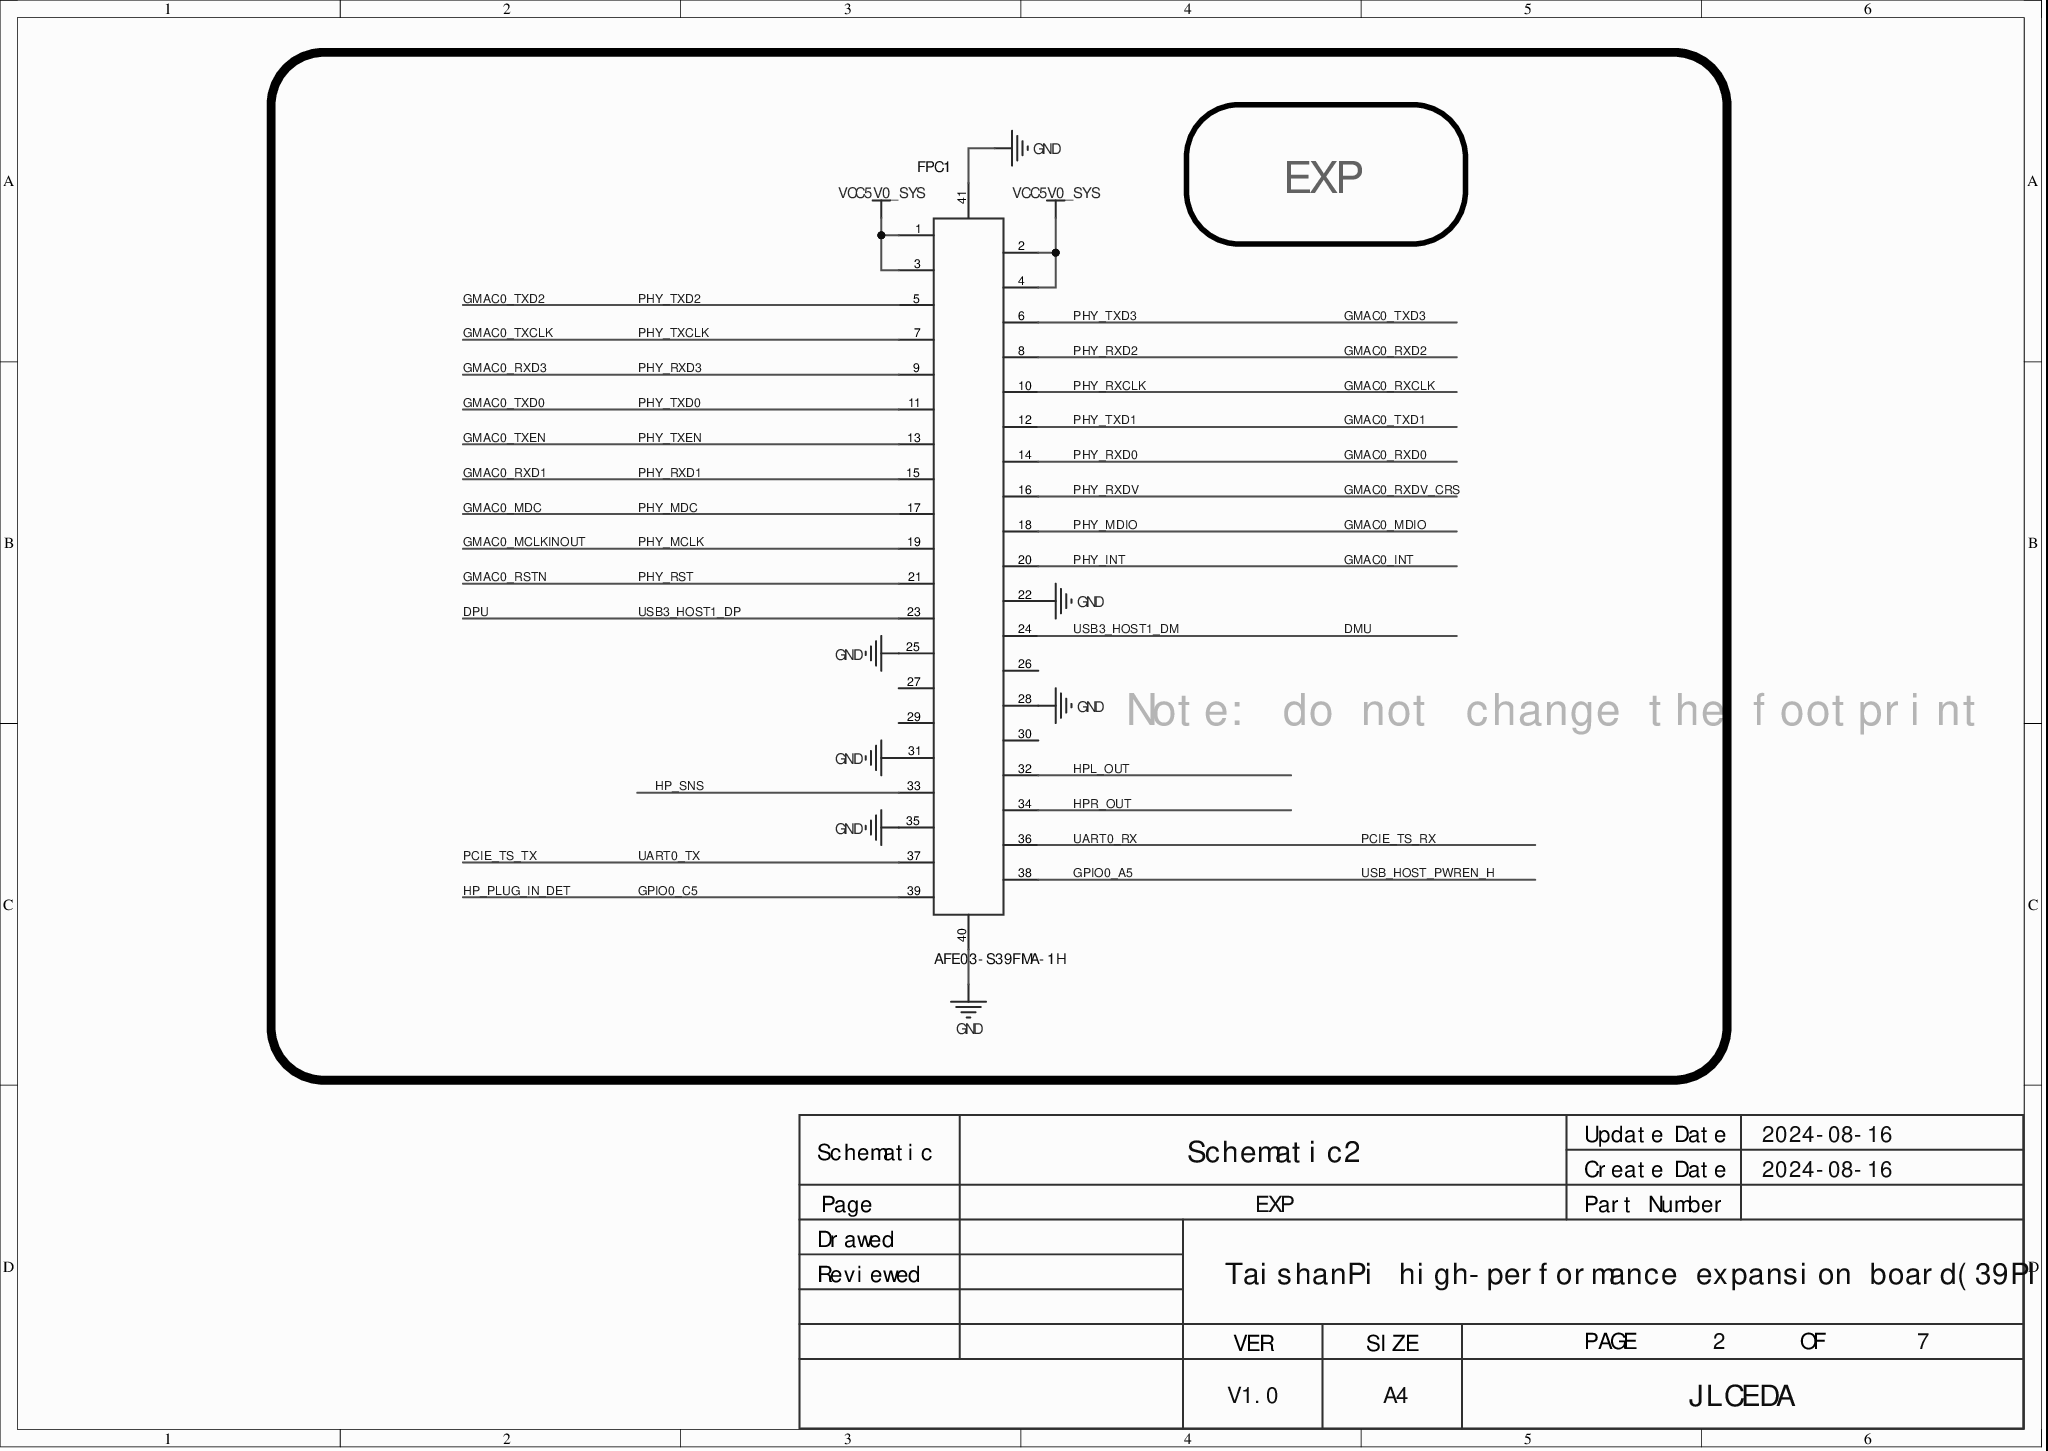
[diagram p0: MISC84334-2.SchDoc]
# Altium project MISC84334.PrjPcb (part 1 of 5)
7 sheets, 209 parts. Net scope: global (net labels, ports and power ports of the same name join across sheets).
Board file: MISC84334.PcbDoc
Sheets:
  MISC84334-2.SchDoc
  MISC84334-3.SchDoc
  MISC84334-4.SchDoc
  MISC84334-5.SchDoc
  MISC84334-6.SchDoc
  MISC84334-7.SchDoc
  MISC84334-8.SchDoc

## Sheet MISC84334-2.SchDoc
size 297 x 210 mm; Symbol: Sheet-Symbol_A4; Company: JLCEDA; Version: V1.0; Page Size: A4; @Project Name: COMPANY_A TaishanPi high-performance expansion board(39PIN); @Page Count: 7; @Update Date: 2024-08-16; @Create Date: 2024-08-16; @Schematic Name: Schematic2; @Page No: 2; @Page Name: EXP; Device: Sheet-Symbol_A4

### Parts
FPC1  AFE03-S39FMA-1H  [FPC-SMD_P0.30-39P_FGS-XJ-H1.0]

### Nets
GND: FPC1.22 FPC1.25 FPC1.28 FPC1.31 FPC1.35 FPC1.40 FPC1.41
VCC5V0_SYS: FPC1.1 FPC1.2 FPC1.3 FPC1.4
DMU: FPC1.24  [also labelled USB3_HOST1_DM]
DPU: FPC1.23  [also labelled USB3_HOST1_DP]
GMAC0_INT: FPC1.20  [also labelled PHY_INT]
GMAC0_MCLKINOUT: FPC1.19  [also labelled PHY_MCLK]
GMAC0_MDC: FPC1.17  [also labelled PHY_MDC]
GMAC0_MDIO: FPC1.18  [also labelled PHY_MDIO]
GMAC0_RSTN: FPC1.21  [also labelled PHY_RST]
GMAC0_RXCLK: FPC1.10  [also labelled PHY_RXCLK]
GMAC0_RXD0: FPC1.14  [also labelled PHY_RXD0]
GMAC0_RXD1: FPC1.15  [also labelled PHY_RXD1]
GMAC0_RXD2: FPC1.8  [also labelled PHY_RXD2]
GMAC0_RXD3: FPC1.9  [also labelled PHY_RXD3]
GMAC0_RXDV_CRS: FPC1.16  [also labelled PHY_RXDV]
GMAC0_TXCLK: FPC1.7  [also labelled PHY_TXCLK]
GMAC0_TXD0: FPC1.11  [also labelled PHY_TXD0]
GMAC0_TXD1: FPC1.12  [also labelled PHY_TXD1]
GMAC0_TXD2: FPC1.5  [also labelled PHY_TXD2]
GMAC0_TXD3: FPC1.6  [also labelled PHY_TXD3]
GMAC0_TXEN: FPC1.13  [also labelled PHY_TXEN]
GPIO0_A5: FPC1.38  [also labelled USB_HOST_PWREN_H]
GPIO0_C5: FPC1.39  [also labelled HP_PLUG_IN_DET]
HP_SNS: FPC1.33
HPL_OUT: FPC1.32
HPR_OUT: FPC1.34
PCIE_TS_RX: FPC1.36  [also labelled UART0_RX]
PCIE_TS_TX: FPC1.37  [also labelled UART0_TX]

Not connected (* = marked no-connect by the designer): FPC1 26 27 29 30

### Notes on the sheet
- EXP
- Note: do not change the footprint
- Update Date
- 2024-08-16
- Schematic
- Page
- Schematic2
- Create Date
- Part Number
- Reviewed
- Drawed
- COMPANY_A TaishanPi high-performance expansion board(39PIN)
- VER
- V1.0
- SIZE
- A4
- PAGE
- 2
- JLCEDA
- OF
- 7

### Library data of the parts
FPC1 = AFE03-S39FMA-1H: Pitch:0.3mm;Contacts:39;Locking:Flip lock;Mounting type:Horizontal SMD;Contact type:Bottom contact;; Manufacturer: JS(钜硕电子); AddInBom: yes; Pitch: 0.3mm; Number of Contacts: 39; FFC, FCB Thickness: 0.2mm; ModelId: 90cc611c06ba4f59bb65cf3349ad002a; ModelTransform: 523.621,133.858,0,180,0,0,0.018,-4.843,0; Symbol: AFE03-S39FMA-1H; Device: AFE03-S39FMA-1H; LCSC Part Name: 0.3mm P数:39 翻盖式 下接; SupplierPart: C262546; ManufacturerPart: AFE03-S39FMA-1H; Supplier Footprint: SMD,P=0.3mm; Datasheet: https://atta.szlcsc.com/upload/public/pdf/source/20180810/C262546_FD07BEB9163FBD4C911947212CF39B0D.pdf; Supplier: LCSC; ConvertToPcb: yes; Locking Feature: Flip lock; Mounting Type: Horizontal SMD; Contact Type: Bottom contact; Height Above Board: 1mm; FootprintName: FPC-SMD_P0.30-39P_FGS-XJ-H1.0; ModelName: FPC-SMD_P0.30-39P_FGS-XJ-H1.0

## Sheet MISC84334-3.SchDoc
size 297 x 210 mm; Symbol: Sheet-Symbol_A4; Company: JLCEDA; Version: V1.0; Page Size: A4; @Project Name: COMPANY_A TaishanPi high-performance expansion board(39PIN); @Page Count: 7; @Update Date: 2024-08-16; @Create Date: 2024-08-16; @Schematic Name: Schematic2; @Page No: 4; @Page Name: FE2.1; Device: Sheet-Symbol_A4
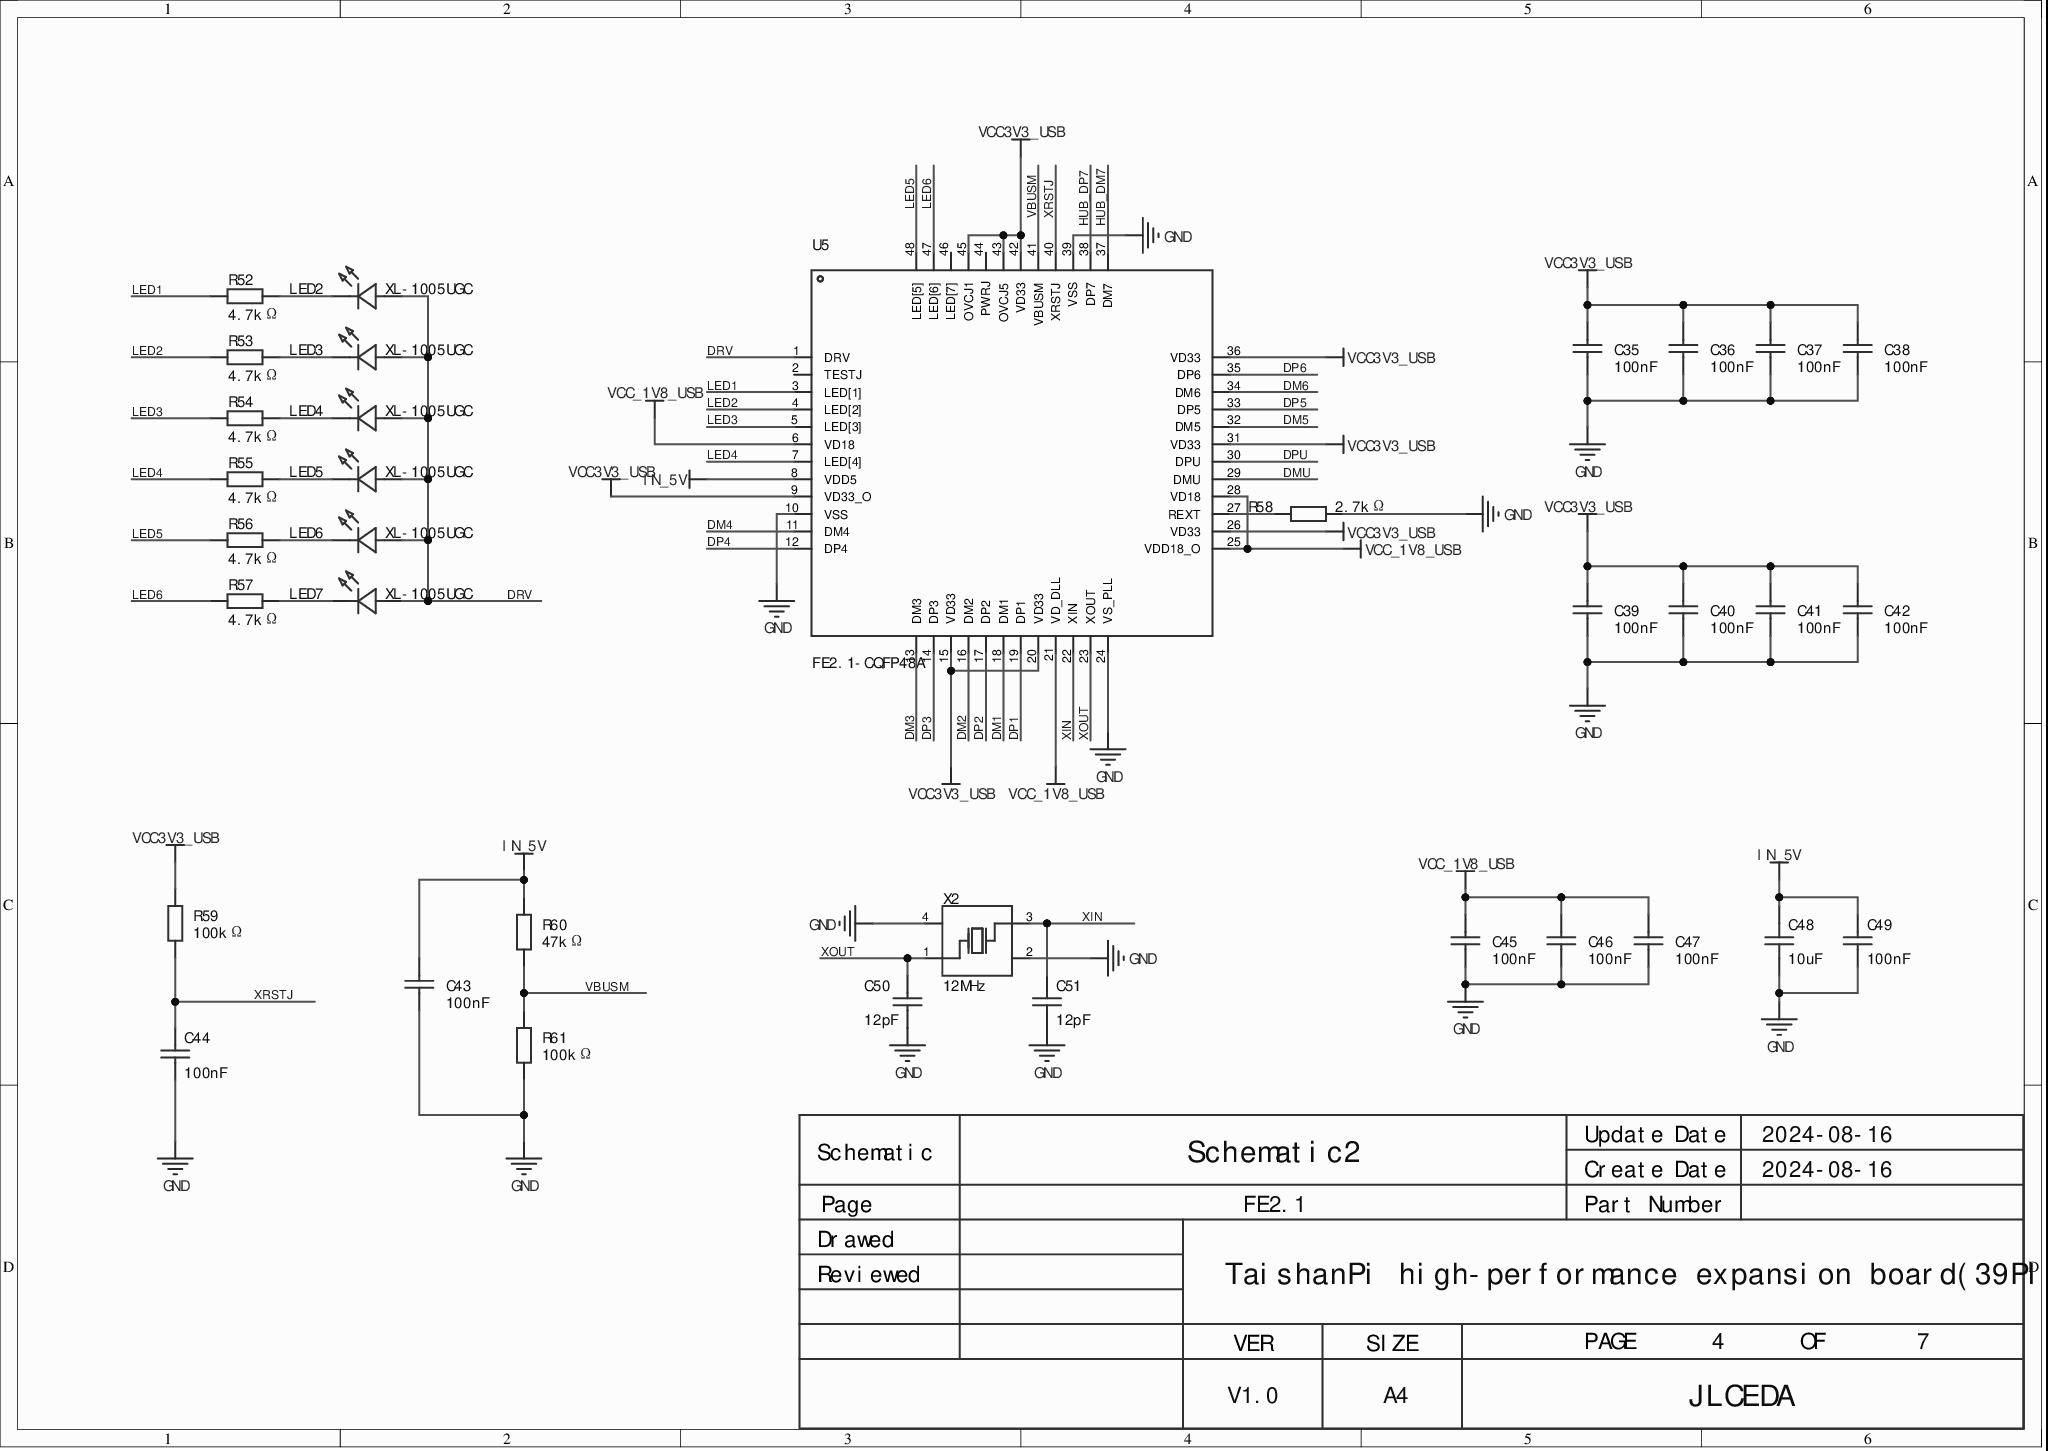
[diagram p1: MISC84334-3.SchDoc]

### Parts
C35  100nF  [R0402]
C36  100nF  [R0402]
C37  100nF  [R0402]
C38  100nF  [R0402]
C39  100nF  [R0402]
C40  100nF  [R0402]
C41  100nF  [R0402]
C42  100nF  [R0402]
C43  100nF  [R0402]
C44  100nF  [R0402]
C45  100nF  [R0402]
C46  100nF  [R0402]
C47  100nF  [R0402]
C48  10uF  [r0603]
C49  100nF  [R0402]
C50  12pF  [R0402]
C51  12pF  [R0402]
LED2  XL-1005UGC  [LED0402-RD_GREEN]
LED3  XL-1005UGC  [LED0402-RD_GREEN]
LED4  XL-1005UGC  [LED0402-RD_GREEN]
LED5  XL-1005UGC  [LED0402-RD_GREEN]
LED6  XL-1005UGC  [LED0402-RD_GREEN]
LED7  XL-1005UGC  [LED0402-RD_GREEN]
R52  4.7kΩ  [R0402]
R53  4.7kΩ  [R0402]
R54  4.7kΩ  [R0402]
R55  4.7kΩ  [R0402]
R56  4.7kΩ  [R0402]
R57  4.7kΩ  [R0402]
R58  2.7kΩ  [R0402]
R59  100kΩ  [R0402]
R60  47kΩ  [R0402]
R61  100kΩ  [R0402]
U5  FE2.1-CQFP48A  [LQFP-48_L7.0-W7.0-P0.50-LS9.0-BL]
X2  12MHz  [OSC-SMD_4P-L3.2-W2.5-BL]

### Nets
GND: C35.1 C36.1 C37.1 C38.1 C39.1 C40.1 C41.1 C42.1 C43.1 C44.1 C45.1 C46.1 C47.1 C48.1 C49.1 C50.1 C51.2 R58.2 R61.1 U5.10(VSS) U5.24(VS_PLL) U5.39(VSS) X2.2(GND) X2.4(GND)
IN_5V: C43.2 C48.2 C49.2 R60.2 U5.8(VDD5)
VCC3V3_USB: C35.2 C36.2 C37.2 C38.2 C39.2 C40.2 C41.2 C42.2 R59.2 U5.9(VD33_O) U5.15(VD33) U5.20(VD33) U5.26(VD33) U5.31(VD33) U5.36(VD33) U5.42(VD33) U5.43(OVCJ5) U5.45(OVCJ1)
VCC_1V8_USB: C45.2 C46.2 C47.2 U5.6(VD18) U5.21(VD_DLL) U5.25(VDD18_O) U5.28(VD18)
DM1: U5.18(DM1)
DM2: U5.16(DM2)
DM3: U5.13(DM3)
DM4: U5.11(DM4)
DM5: U5.32(DM5)
DM6: U5.34(DM6)
DMU: U5.29(DMU)
DP1: U5.19(DP1)
DP2: U5.17(DP2)
DP3: U5.14(DP3)
DP4: U5.12(DP4)
DP5: U5.33(DP5)
DP6: U5.35(DP6)
DPU: U5.30(DPU)
DRV: LED2.2(A) LED3.2(A) LED4.2(A) LED5.2(A) LED6.2(A) LED7.2(A) U5.1(DRV)
HUB_DM7: U5.37(DM7)
HUB_DP7: U5.38(DP7)
LED1: R52.2 U5.3(LED[1])
LED2: R53.2 U5.4(LED[2])
LED3: R54.2 U5.5(LED[3])
LED4: R55.2 U5.7(LED[4])
LED5: R56.2 U5.48(LED[5])
LED6: R57.2 U5.47(LED[6])
VBUSM: R60.1 R61.2 U5.41(VBUSM)
XIN: C51.1 U5.22(XIN) X2.3(OSC2)
XOUT: C50.2 U5.23(XOUT) X2.1(OSC1)
XRSTJ: C44.2 R59.1 U5.40(XRSTJ)
NetLED2_1: LED2.1(K) R52.1
NetLED3_1: LED3.1(K) R53.1
NetLED4_1: LED4.1(K) R54.1
NetLED5_1: LED5.1(K) R55.1
NetLED6_1: LED6.1(K) R56.1
NetLED7_1: LED7.1(K) R57.1
NetR58_1: R58.1 U5.27(REXT)

Not connected (* = marked no-connect by the designer): U5 2(TESTJ)* 44(PWRJ)* 46(LED[7])*

### Notes on the sheet
- Update Date
- 2024-08-16
- Schematic
- Page
- Schematic2
- FE2.1
- Create Date
- Part Number
- Reviewed
- Drawed
- COMPANY_A TaishanPi high-performance expansion board(39PIN)
- VER
- V1.0
- SIZE
- A4
- PAGE
- 4
- JLCEDA
- OF
- 7

### Library data of the parts
C35-C47 C49 = CL05B104KO5NNNC: Capacitance:100nF;Tolerance:±10%;Rated voltage:16V;Dielectric(Temp. coefficient):X7R;; Manufacturer: SAMSUNG(三星); AddInBom: yes; ModelId: 36a51122f27c49738f86b3bfa98863e0; ModelName: C0402_L1.0-W0.5-H0.5; ModelTransform: 39.37,19.685,0,0,0,0,0,0,0; Tolerance: ±10%; Voltage Rated: 16V; Temperature Coefficient: X7R; Symbol: CL05B104KO5NNNC; Device: CL05B104KO5NNNC; LCSC Part Name: 100nF ±10% 16V; SupplierPart: C1525; ManufacturerPart: CL05B104KO5NNNC; Supplier Footprint: 0402; JLCPCB Part Class: Basic library; Datasheet: https://atta.szlcsc.com/upload/public/pdf/source/20160103/1457707674891.pdf; Supplier: LCSC; ConvertToPcb: yes; FootprintName: R0402; Value: 100nF
C48 = 0603X106M100CT: Capacitance:10uF;Tolerance:±20%;Rated voltage:10V;Dielectric(Temp. coefficient):X5R;; Manufacturer: Walsin(华新科); AddInBom: yes; ModelId: ac125912035d415993ca9572d50418b1; ModelName: C0603_L1.6-W0.8-H0.8; ModelTransform: 62.992,31.496,0,0,0,0,0,0,0; Tolerance: ±20%; Voltage Rated: 10V; Temperature Coefficient: X5R; Symbol: 0603X106M100; Device: 0603X106M100CT; LCSC Part Name: 10uF ±20% 10V; SupplierPart: C89283; ManufacturerPart: 0603X106M100CT; Supplier Footprint: 0603; JLCPCB Part Class: Extended library; Datasheet: https://atta.szlcsc.com/upload/public/pdf/source/20161226/1482720147964.pdf; Supplier: LCSC; ConvertToPcb: yes; FootprintName: r0603; Value: 10uF
C50 C51 = 0402CG120J500NT: Capacitance:12pF;Tolerance:±5%;Rated voltage:50V;Dielectric(Temp. coefficient):C0G;; Manufacturer: FH(风华); Symbol: 0402CG200J500NT; Capacitance: 20pF; AddInBom: yes; ModelId: 36a51122f27c49738f86b3bfa98863e0; ModelName: C0402_L1.0-W0.5-H0.5; ModelTransform: 39.37,19.685,0,0,0,0,0,0,0; Tolerance: ±5%; Voltage Rated: 50V; Temperature Coefficient: C0G; JLCPCB Part Class: Basic Part; Device: 0402CG120J500NT; Supplier: LCSC; Manufacturer Part: 0402CG120J500NT; Supplier Part: C1547; LCSC Part Name: 12pF ±5% 50V; Supplier Footprint: 0402; Datasheet: https://atta.szlcsc.com/upload/public/pdf/source/20200305/C486355_26A10D38EF8C2A5C37091D0039909270.pdf; ConvertToPcb: yes; FootprintName: R0402; Value: 12pF
LED2-LED7 = XL-1005UGC: Emitting color:Emerald green;Dominant wavelength:516nm;Color temp.:-;Power:80mW;Mounting:Top mount;; Manufacturer: XINGLIGHT(成兴光); Symbol: XL-1005UGC_C2856703; AddInBom: yes; ModelId: 080bb9bd520f4b34ac21e218e7b036d6; ModelName: LED0402_L1.0-W0.5-H0.2; ModelTransform: 40.1574,19.685,0,0,0,0,0,-0.0005,0; Lens Color: Water clear; Dominant Wavelength: 516nm; Peak Wavelength: 531nm; Forward Current: 25mA; Power Dissipation: 80mW; Viewing Angle: 120°; Device: XL-1005UGC; LCSC Part Name: 正贴; SupplierPart: C2856703; ManufacturerPart: XL-1005UGC; Supplier Footprint: 0402; Datasheet: https://atta.szlcsc.com/upload/public/pdf/source/20221102/FF8D6BC2225363A60A01D46BB802F217.pdf; Supplier: LCSC; ConvertToPcb: yes; FootprintName: LED0402-RD_GREEN; Emitted Color: Emerald green; Color Temperature: -; Mounting Sytle: Top mount; Operating Temperature: -30℃~+85℃
R52-R57 = 0402WGF4701TCE: Resistor type:Thick film resistor;Resistance:4.7kΩ;Tolerance:±1%;Power:62.5mW;; Manufacturer: UNI-ROYAL(厚声); AddInBom: yes; ModelId: 671aefced39d4c318694bba8bd8efd39; ModelName: R0402_L1.0-W0.5-H0.5; ModelTransform: 39.37,19.685,0,0,0,0,0,0.0005,0; Tolerance: ±1%; Power(Watts): 62.5mW; Temperature Coefficient: ±100ppm/℃; Overload Voltage (Max): 50V; Symbol: 0402WGF4701TCE; Device: 0402WGF4701TCE; Supplier: LCSC; Manufacturer Part: 0402WGF4701TCE; Supplier Part: C25900; Value: 4.7kΩ; JLCPCB Part Class: Basic library; LCSC Part Name: 4.7kΩ ±1% 62.5mW; Supplier Footprint: 0402; Datasheet: https://atta.szlcsc.com/upload/public/pdf/source/20200306/C422600_1E6D84923E4A46A82E41ADD87F860B5C.pdf; ConvertToPcb: yes; FootprintName: R0402; Type: Thick film resistor; Operating Temperature Range: -55℃~+155℃
R58 = RC0402FR-072K7L: Resistor type:Thick film resistor;Resistance:2.7kΩ;Tolerance:±1%;Power:62.5mW;; Manufacturer: YAGEO(国巨); AddInBom: yes; ModelId: 671aefced39d4c318694bba8bd8efd39; ModelName: R0402_L1.0-W0.5-H0.5; ModelTransform: 39.37,19.685,0,0,0,0,0,0.0005,0; Tolerance: ±1%; Power(Watts): 62.5mW; Temperature Coefficient: ±100ppm/℃; Overload Voltage (Max): 50V; Symbol: RC0402FR-072K7L; Device: RC0402FR-072K7L; LCSC Part Name: 2.7kΩ ±1% 62.5mW; SupplierPart: C138017; ManufacturerPart: RC0402FR-072K7L; Supplier Footprint: 0402; Datasheet: https://atta.szlcsc.com/upload/public/pdf/source/20171107/C138017_15100516423651096944.pdf; Supplier: LCSC; ConvertToPcb: yes; FootprintName: R0402; Type: Thick film resistor; Value: 2.7kΩ; Operating Temperature Range: -55℃~+155℃
R59 R61 = 0402WGF1003TCE: Resistor type:Thick film resistor;Resistance:100kΩ;Tolerance:±1%;Power:62.5mW;Temp. coefficient:±100ppm/℃;Max working voltage:50V;Operating temperature:-55℃~+155℃;; Manufacturer: UNI-ROYAL(厚声); AddInBom: yes; ModelId: 671aefced39d4c318694bba8bd8efd39; ModelName: R0402_L1.0-W0.5-H0.5; ModelTransform: 39.37,19.685,0,0,0,0,0,0.0005,0; Tolerance: ±1%; Power(Watts): 62.5mW; Overload Voltage (Max): 50V; Symbol: 0402WGF1003TCE; Device: 0402WGF1003TCE; LCSC Part Name: 100kΩ ±1% 62.5mW; SupplierPart: C25741; ManufacturerPart: 0402WGF1003TCE; Supplier Footprint: 0402; JLCPCB Part Class: Basic Part; Datasheet: https://atta.szlcsc.com/upload/public/pdf/source/20200306/C422600_1E6D84923E4A46A82E41ADD87F860B5C.pdf; Supplier: LCSC; ConvertToPcb: yes; FootprintName: R0402; Type: Thick film resistor; Value: 100kΩ; Temperature Coefficient: ±100ppm/℃; Operating Temperature Range: -55℃~+155℃
R60 = 0402WGF4702TCE: Resistor type:Thick film resistor;Resistance:47kΩ;Tolerance:±1%;Power:62.5mW;; Manufacturer: UNI-ROYAL(厚声); AddInBom: yes; ModelId: 671aefced39d4c318694bba8bd8efd39; ModelName: R0402_L1.0-W0.5-H0.5; ModelTransform: 39.37,19.685,0,0,0,0,0,0.0005,0; Tolerance: ±1%; Power(Watts): 62.5mW; Temperature Coefficient: ±100ppm/℃; Overload Voltage (Max): 50V; Symbol: 0402WGF4702TCE; Device: 0402WGF4702TCE; LCSC Part Name: 47kΩ ±1% 62.5mW; SupplierPart: C25792; ManufacturerPart: 0402WGF4702TCE; Supplier Footprint: 0402; Datasheet: https://atta.szlcsc.com/upload/public/pdf/source/20200306/C422600_1E6D84923E4A46A82E41ADD87F860B5C.pdf; Supplier: LCSC; ConvertToPcb: yes; FootprintName: R0402; Type: Thick film resistor; Value: 47kΩ; Operating Temperature Range: -55℃~+155℃
U5 = FE2.1-CQFP48A: Type:-;Protocol:-;Drivers/receivers:-;Data rate:-;; Manufacturer: TERMINUS; Symbol: FE2.1; AddInBom: yes; ModelId: 093be70396ff421eb2cdb946d5311efc; ModelName: LQFP-48_L7.0-W7.0-H1.4-LS9.0-P0.50; ModelTransform: 354.331,354.331,0,0,0,0,0,0,0; Device: FE2.1-CQFP48A; LCSC Part Name: FE2.1-CQFP48A; SupplierPart: C39693; ManufacturerPart: FE2.1-CQFP48A; Supplier Footprint: LQFP-48(7x7); Datasheet: https://atta.szlcsc.com/upload/public/pdf/source/20220804/15245222ED887981AE0D8A621FDC31A4.pdf; Supplier: LCSC; ConvertToPcb: yes; FootprintName: LQFP-48_L7.0-W7.0-P0.50-LS9.0-BL; Type: -; Protocol: -; Number of Drivers/Receivers: -; Data Rate: -; Supply Voltage: -
X2 = X322512MSB4SI: Frequency:12MHz;Frequency tolerance:±10ppm;Load capacitance:20pF;; Manufacturer: YXC(扬兴晶振); AddInBom: yes; ModelId: ae22b8d143894765bc8100c37cb6356f; ModelName: OSC-SMD_4P-L3.2-W2.5-H1.0; ModelTransform: 125.984,98.425,0,0,0,0,0,0,0; Crystal Type: SMD passive crystal; Frequency Tolerance: ±10ppm; Frequency Stability: ±30ppm; Load Capacitance: 20pF; Symbol: X322512MSB4SI; Device: X322512MSB4SI; LCSC Part Name: 12MHz ±10ppm 20pF YSX321SL; SupplierPart: C9002; ManufacturerPart: X322512MSB4SI; Supplier Footprint: SMD3225-4P; Datasheet: https://atta.szlcsc.com/upload/public/pdf/source/20210329/C112971_1F611BDC486E193C1706F6D8EB5AA189.pdf; Supplier: LCSC; ConvertToPcb: yes; FootprintName: OSC-SMD_4P-L3.2-W2.5-BL; Value: 12MHz; Operating Temperature: -40℃~+85℃

## Sheet MISC84334-4.SchDoc
size 297 x 210 mm; Symbol: Sheet-Symbol_A4; Company: JLCEDA; Version: V1.0; Page Size: A4; @Project Name: COMPANY_A TaishanPi bottom 39Pin_Hub2.0_Ethernet expansion board 0419 revision; @Page Count: 7; @Update Date: 2024-08-16; @Create Date: 2024-08-16; @Schematic Name: Schematic; @Page No: 3; @Page Name: GMAC; Device: Sheet-Symbol_A4
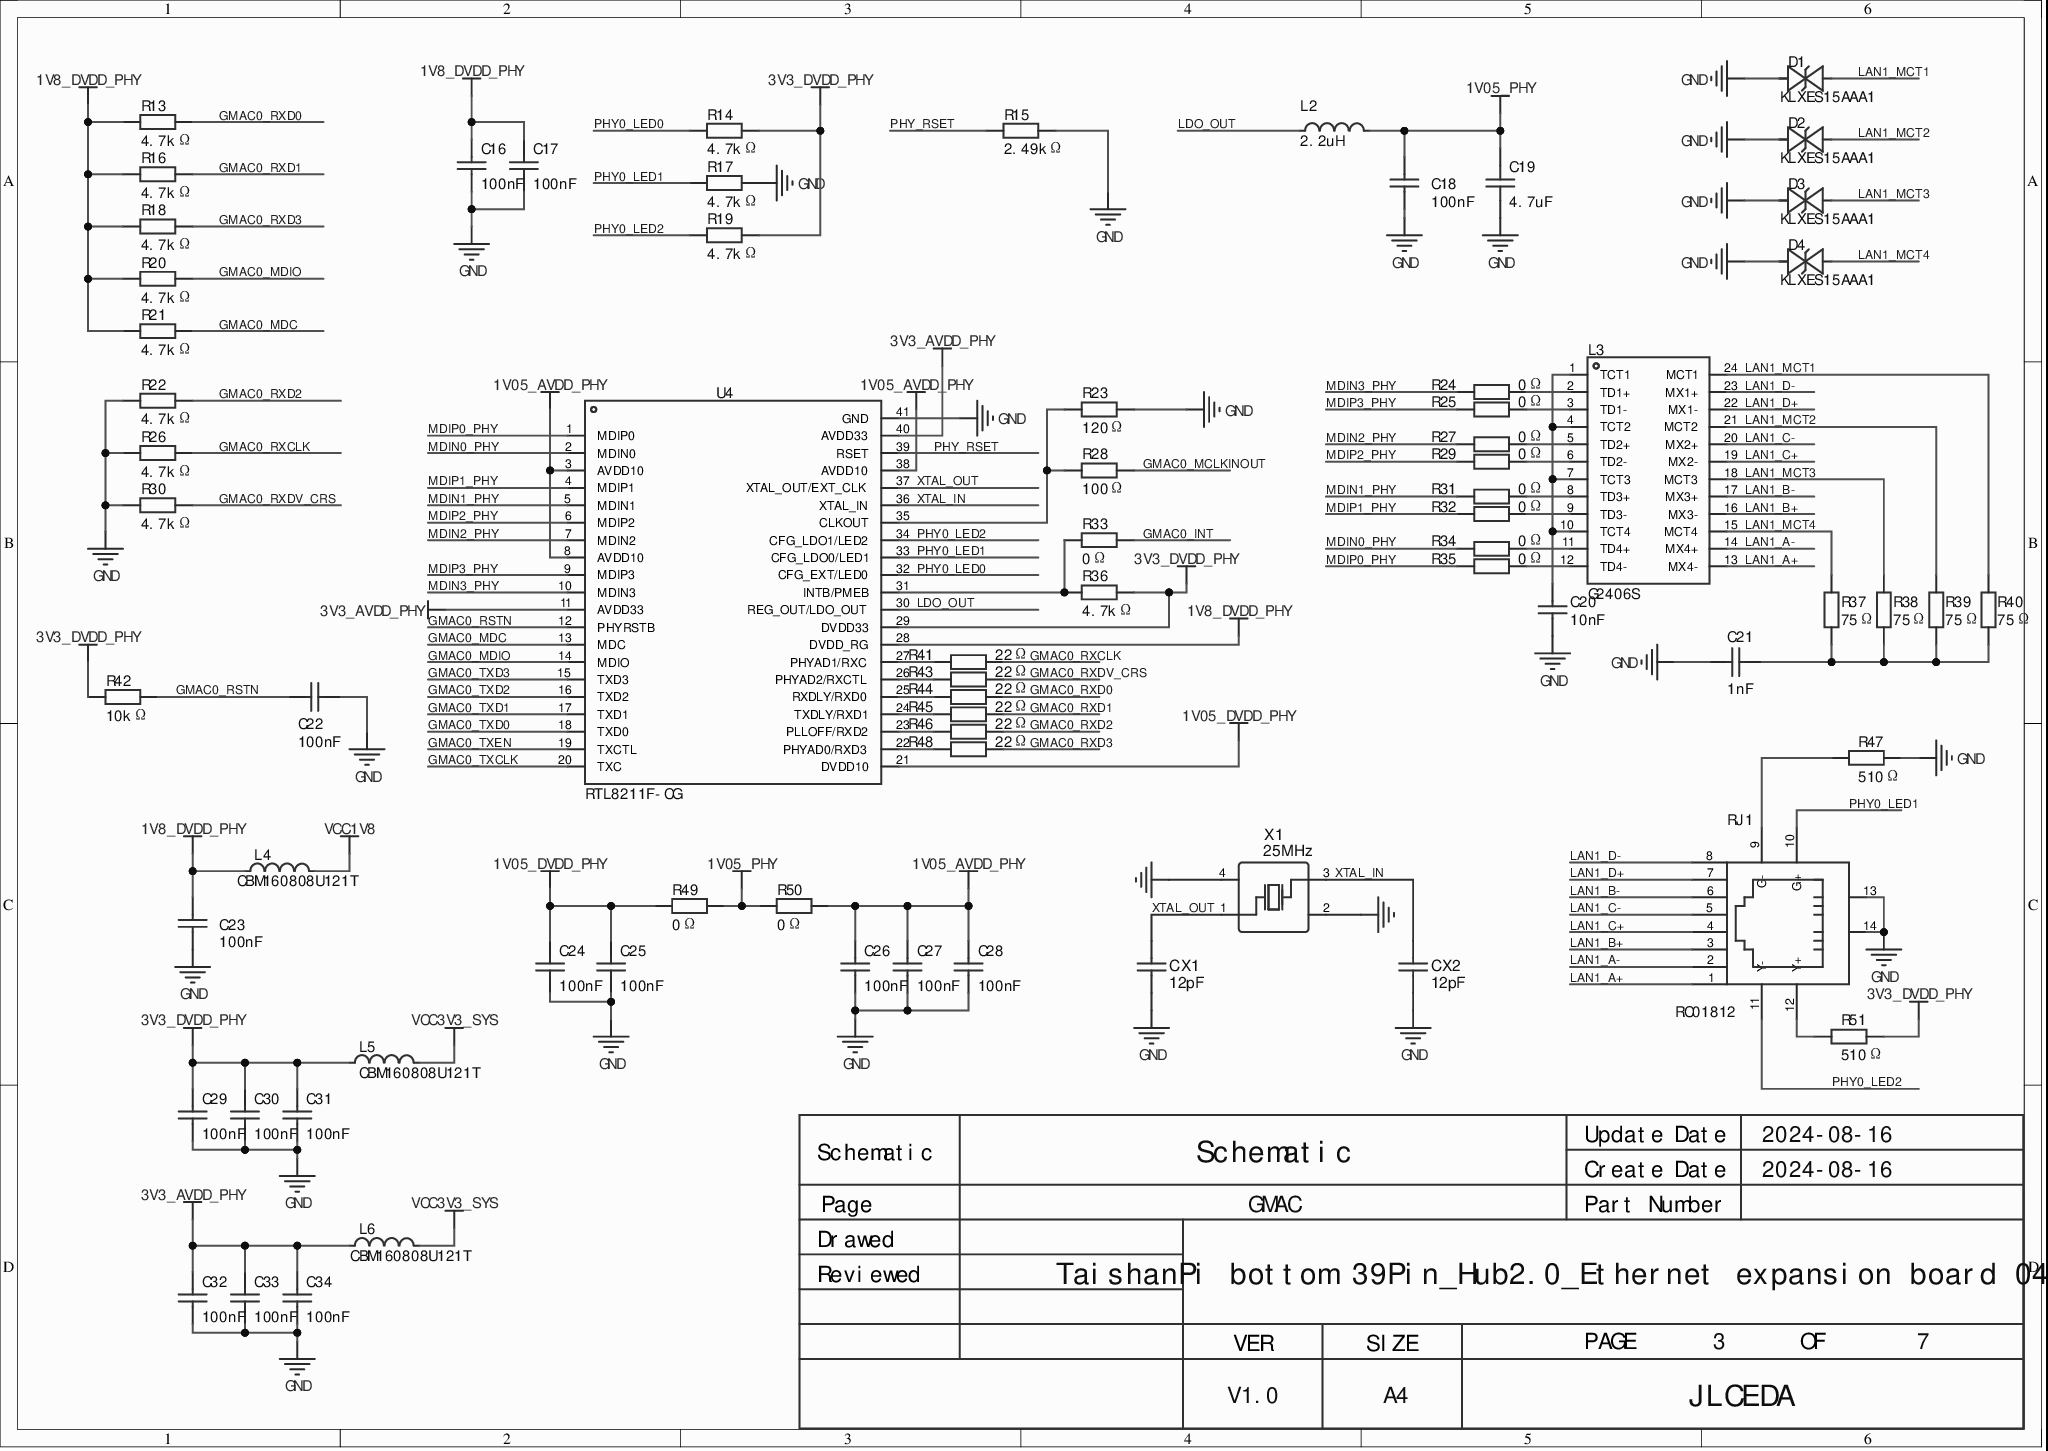
[diagram p2: MISC84334-4.SchDoc]

### Parts
C16  100nF  [R0402]